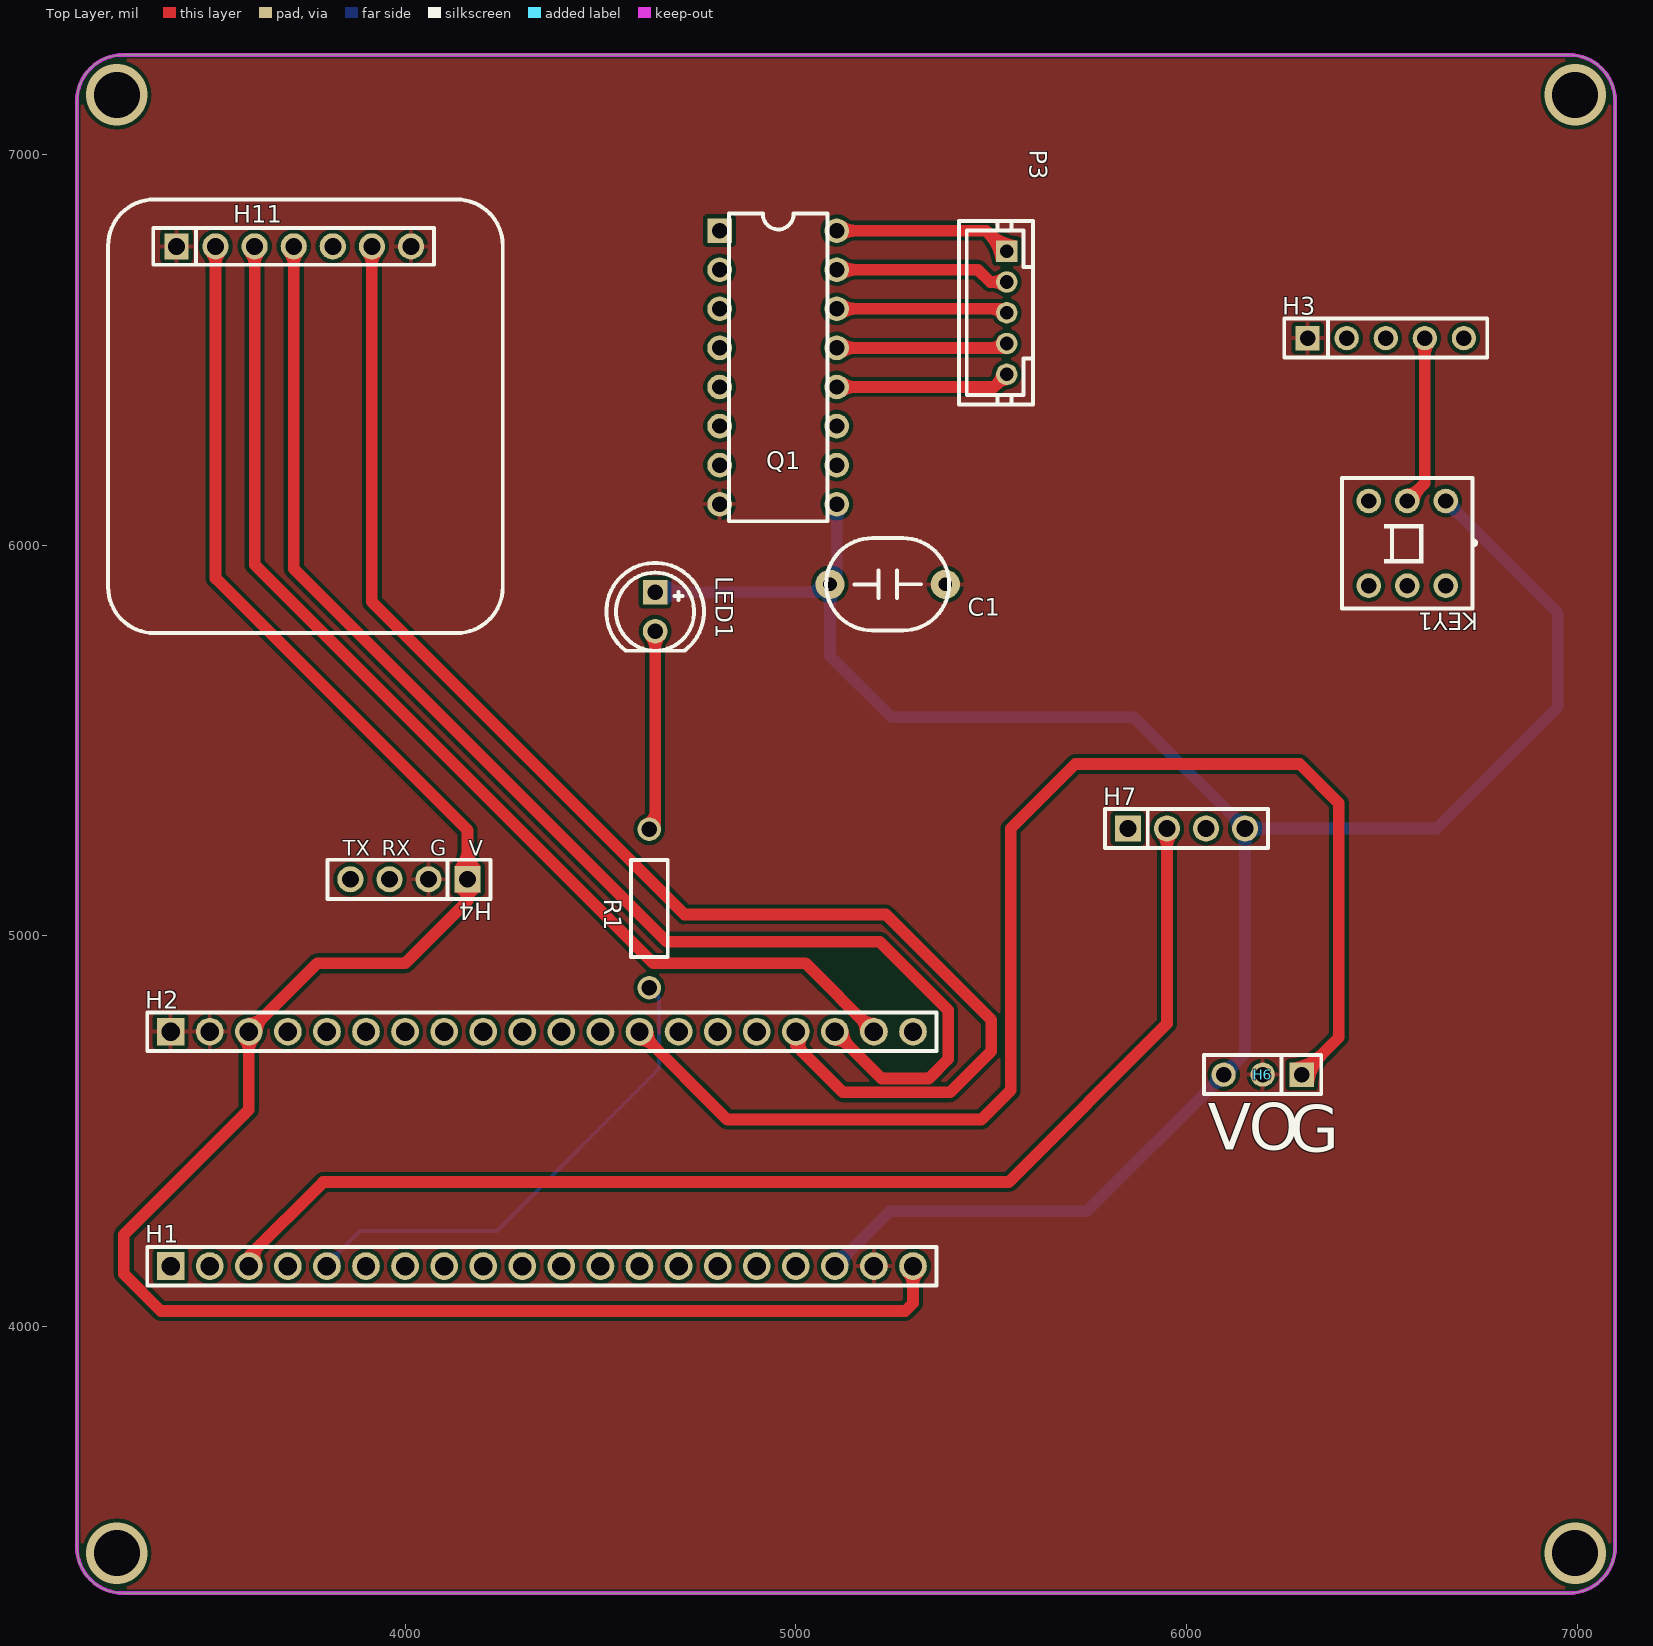
[diagram p0: Top Layer view]
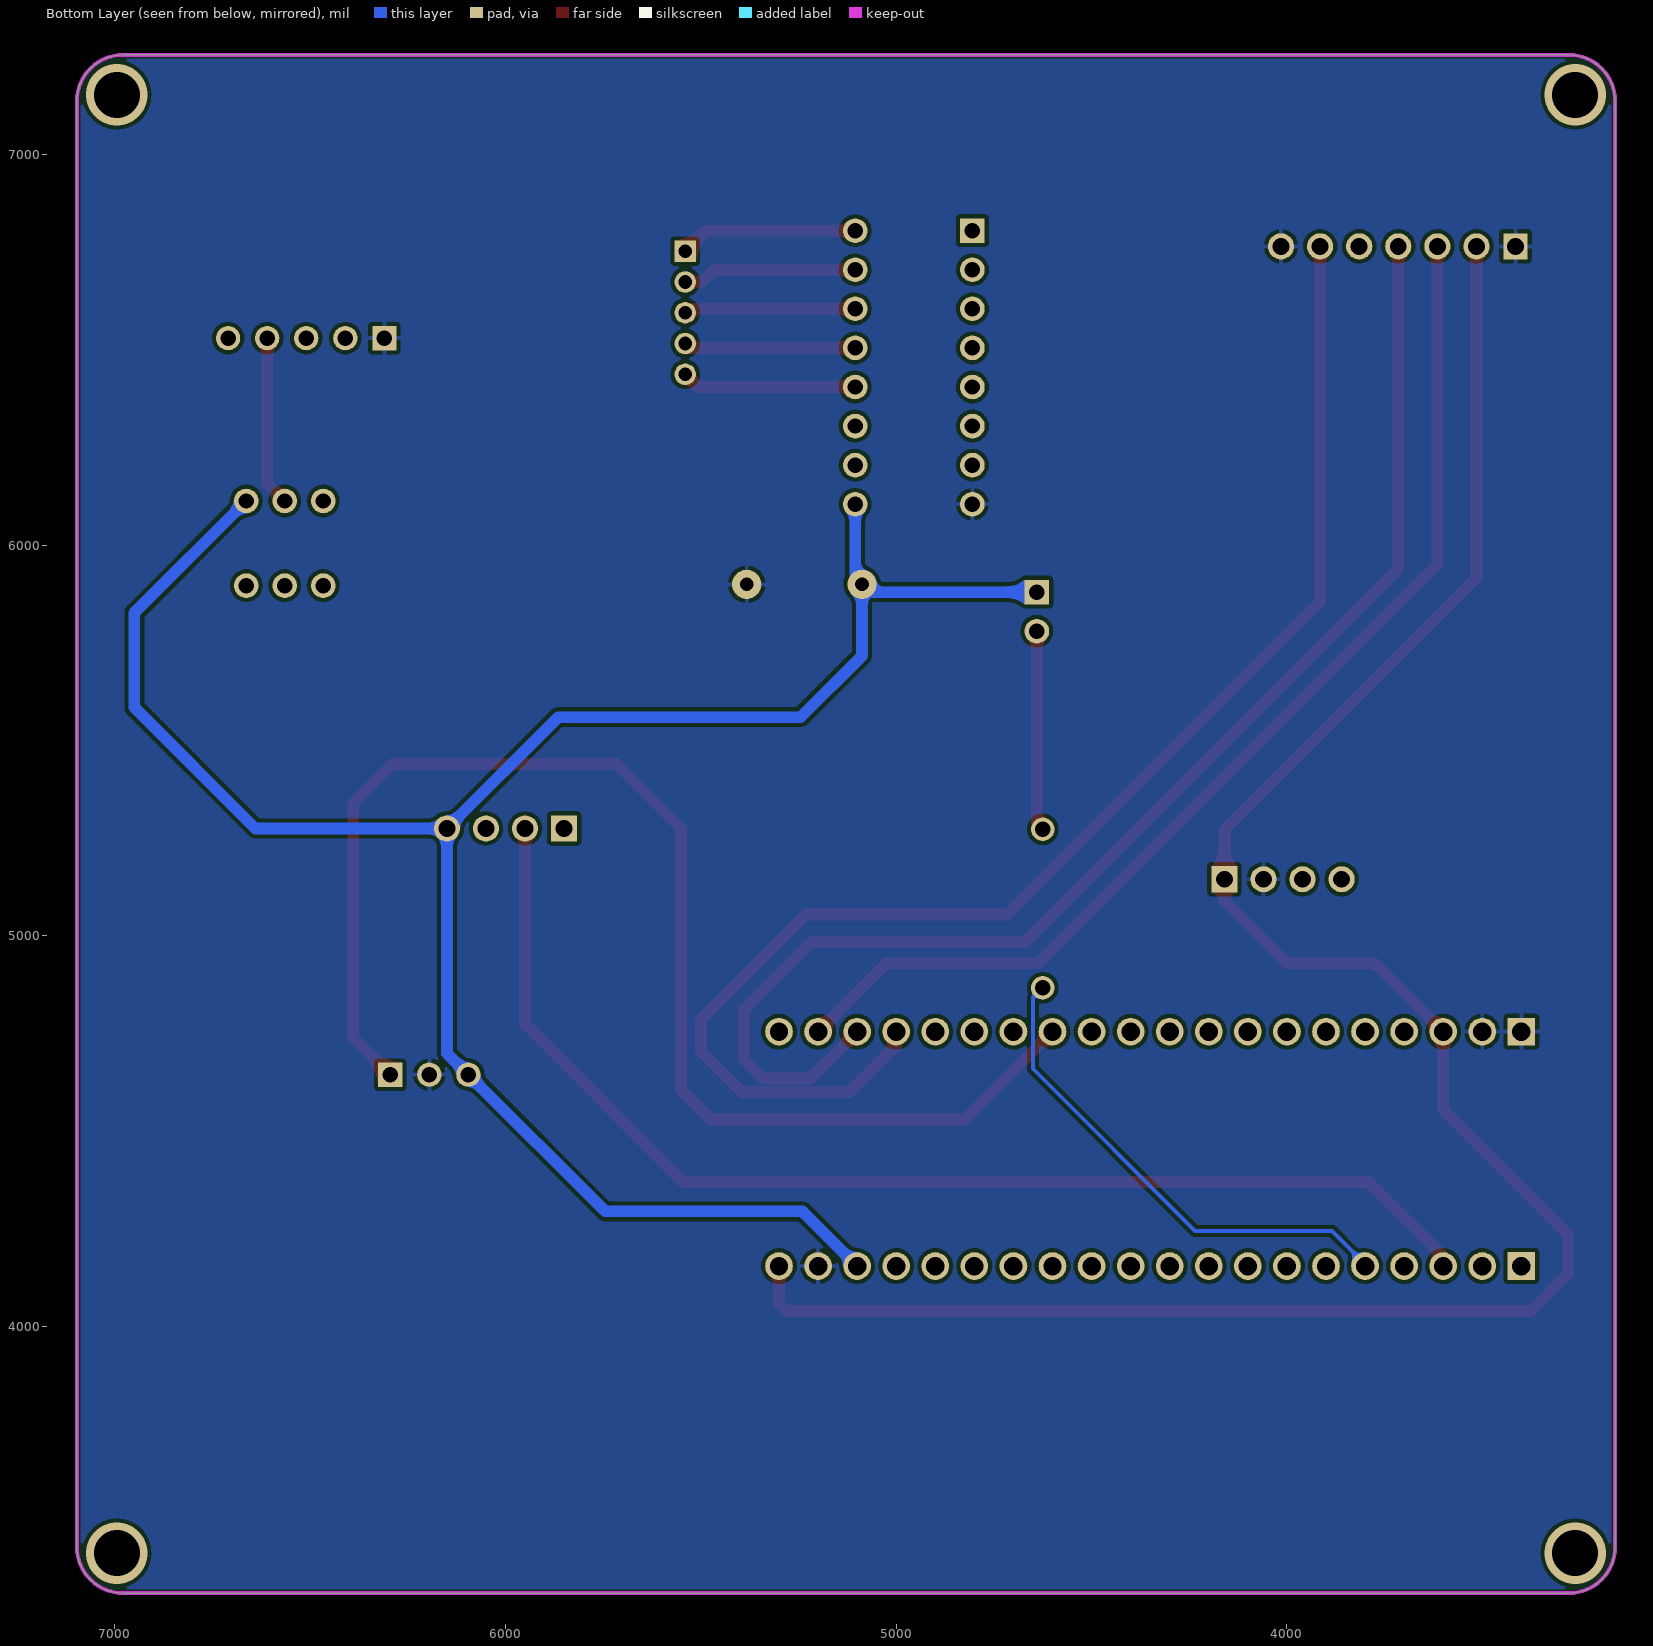
[diagram p1: Bottom Layer view, seen from below]
# Altium PCB MISC89064.pcbdoc
Units mil, origin at the board's own origin, x right, y up, seen from the top; angles counter-clockwise.
Board outline 3937.01 x 3937.01 mil, 2 copper layers (Top Layer, Bottom Layer), stack 62.206 mil thick; 13 components, 49 nets, 96 pads, 4 vias.

## Layer stack, top to bottom
Top Solder Mask Layer: solder mask 0.394, Dk 3.3
Top Layer: signal copper 1.379
Dielectric1: surface 59.449, FR4, Dk 4.5
Bottom Layer: signal copper 1.378
Bottom Solder Mask Layer: solder mask 0.394, Dk 3.3

## Board outline
3278.11,7255 ccw(c3278.11,7136.89) 3160,7136.89 3160,3436.1 ccw(c3278.11,3436.1) 3278.11,3317.99 6978.9,3317.99 ccw(c6978.9,3436.1) 7097.01,3436.1 7097.01,7136.89 ccw(c6978.9,7136.89) 6978.9,7255

## Design rules (kind name [scope] priority, off if disabled: settings)
BoardOutlineClearance copperThickness2oz_1 [All] p2 off: genericclearance=7.99 ignorepadtopadclearanceinfootprint=FALSE except(0: Arc-SplitContinuation Track-SplitContinuation SMDPad-SplitContinuation THPad-SplitContinuation Via-SplitContinuation Fill-SplitContinuation Region-SplitContinuation Poly-SplitContinuation Text-SplitContinuation Hole-SplitContinuation; 5.98: SMDPad-CutoutEdge THPad-CutoutEdge Via-CutoutEdge Fill-CutoutEdge Region-CutoutEdge Text-CutoutEdge Hole-CutoutEdge; 10: Poly-OutlineEdge Poly-CutoutEdge; 11.81: Arc-OutlineEdge Track-OutlineEdge SMDPad-OutlineEdge THPad-OutlineEdge Via-OutlineEdge Fill-OutlineEdge Region-OutlineEdge Text-OutlineEdge Hole-OutlineEdge Arc-CutoutEdge Track-CutoutEdge)
BoardOutlineClearance Plane_innerPlane_1 [All] p4 off: genericclearance=4.02 ignorepadtopadclearanceinfootprint=FALSE except(0: Arc-SplitContinuation Track-SplitContinuation SMDPad-SplitContinuation THPad-SplitContinuation Via-SplitContinuation Fill-SplitContinuation Region-SplitContinuation Poly-SplitContinuation Text-SplitContinuation Hole-SplitContinuation; 5.98: SMDPad-CutoutEdge THPad-CutoutEdge Via-CutoutEdge Fill-CutoutEdge Region-CutoutEdge Text-CutoutEdge Hole-CutoutEdge; 10: Poly-OutlineEdge Poly-CutoutEdge; 11.81: Arc-OutlineEdge Track-OutlineEdge SMDPad-OutlineEdge THPad-OutlineEdge Via-OutlineEdge Fill-OutlineEdge Region-OutlineEdge Text-OutlineEdge Hole-OutlineEdge Arc-CutoutEdge Track-CutoutEdge)
BoardOutlineClearance Copper_copperRegion_1 [All] p6 off: genericclearance=4.02 ignorepadtopadclearanceinfootprint=FALSE except(0: Arc-SplitContinuation Track-SplitContinuation SMDPad-SplitContinuation THPad-SplitContinuation Via-SplitContinuation Fill-SplitContinuation Region-SplitContinuation Poly-SplitContinuation Text-SplitContinuation Hole-SplitContinuation; 5.98: SMDPad-CutoutEdge THPad-CutoutEdge Via-CutoutEdge Fill-CutoutEdge Region-CutoutEdge Text-CutoutEdge Hole-CutoutEdge; 10: Poly-OutlineEdge Poly-CutoutEdge; 11.81: Arc-OutlineEdge Track-OutlineEdge SMDPad-OutlineEdge THPad-OutlineEdge Via-OutlineEdge Fill-OutlineEdge Region-OutlineEdge Text-OutlineEdge Hole-OutlineEdge Arc-CutoutEdge Track-CutoutEdge)
BoardOutlineClearance copperThickness1oz_1 [All] p8: genericclearance=4.02 ignorepadtopadclearanceinfootprint=FALSE except(0: Arc-SplitContinuation Track-SplitContinuation SMDPad-SplitContinuation THPad-SplitContinuation Via-SplitContinuation Fill-SplitContinuation Region-SplitContinuation Poly-SplitContinuation Text-SplitContinuation Hole-SplitContinuation; 5.98: SMDPad-CutoutEdge THPad-CutoutEdge Via-CutoutEdge Fill-CutoutEdge Region-CutoutEdge Text-CutoutEdge Hole-CutoutEdge; 10: Poly-OutlineEdge Poly-CutoutEdge; 11.81: Arc-OutlineEdge Track-OutlineEdge SMDPad-OutlineEdge THPad-OutlineEdge Via-OutlineEdge Fill-OutlineEdge Region-OutlineEdge Text-OutlineEdge Hole-OutlineEdge Arc-CutoutEdge Track-CutoutEdge)
Clearance copperThickness2oz [All] p1 off: gap=7.99 ignorepadtopadclearanceinfootprint=FALSE except(5.98: SMDPad-Track SMDPad-SMDPad THPad-Track SMDPad-THPad THPad-THPad Track-Via SMDPad-Via THPad-Via Via-Via Fill-Track Region-Track Fill-SMDPad Region-SMDPad Fill-THPad Region-THPad Fill-Via Region-Via Fill-Fill Fill-Region Region-Region Arc-Track Arc-SMDPad Arc-THPad Arc-Via Fill-Arc Region-Arc Arc-Arc Text-Track SMDPad-Text Text-THPad Text-Via Fill-Text Region-Text Arc-Text Text-Text Hole-Track Hole-SMDPad Hole-THPad Hole-Via Fill-Hole Region-Hole Hole-Arc Hole-Text; 10: Poly-Track Poly-SMDPad Poly-THPad Poly-Via Poly-Fill Poly-Region Poly-Poly Poly-Arc Poly-Text Poly-Hole)
Clearance Plane_innerPlane [All] p3 off: gap=4.02 ignorepadtopadclearanceinfootprint=FALSE except(5.98: SMDPad-Track SMDPad-SMDPad THPad-Track SMDPad-THPad THPad-THPad Track-Via SMDPad-Via THPad-Via Via-Via Fill-Track Region-Track Fill-SMDPad Region-SMDPad Fill-THPad Region-THPad Fill-Via Region-Via Fill-Fill Fill-Region Region-Region Arc-Track Arc-SMDPad Arc-THPad Arc-Via Fill-Arc Region-Arc Arc-Arc Text-Track SMDPad-Text Text-THPad Text-Via Fill-Text Region-Text Arc-Text Text-Text Hole-Track Hole-SMDPad Hole-THPad Hole-Via Fill-Hole Region-Hole Hole-Arc Hole-Text; 10: Poly-Track Poly-SMDPad Poly-THPad Poly-Via Poly-Fill Poly-Region Poly-Poly Poly-Arc Poly-Text Poly-Hole)
Clearance Copper_copperRegion [All] p5 off: gap=4.02 ignorepadtopadclearanceinfootprint=FALSE except(5.98: SMDPad-Track SMDPad-SMDPad THPad-Track SMDPad-THPad THPad-THPad Track-Via SMDPad-Via THPad-Via Via-Via Fill-Track Region-Track Fill-SMDPad Region-SMDPad Fill-THPad Region-THPad Fill-Via Region-Via Fill-Fill Fill-Region Region-Region Arc-Track Arc-SMDPad Arc-THPad Arc-Via Fill-Arc Region-Arc Arc-Arc Text-Track SMDPad-Text Text-THPad Text-Via Fill-Text Region-Text Arc-Text Text-Text Hole-Track Hole-SMDPad Hole-THPad Hole-Via Fill-Hole Region-Hole Hole-Arc Hole-Text; 10: Poly-Track Poly-SMDPad Poly-THPad Poly-Via Poly-Fill Poly-Region Poly-Poly Poly-Arc Poly-Text Poly-Hole)
Clearance copperThickness1oz [All] p7: gap=4.02 ignorepadtopadclearanceinfootprint=FALSE except(5.98: SMDPad-Track SMDPad-SMDPad THPad-Track SMDPad-THPad THPad-THPad Track-Via SMDPad-Via THPad-Via Via-Via Fill-Track Region-Track Fill-SMDPad Region-SMDPad Fill-THPad Region-THPad Fill-Via Region-Via Fill-Fill Fill-Region Region-Region Arc-Track Arc-SMDPad Arc-THPad Arc-Via Fill-Arc Region-Arc Arc-Arc Text-Track SMDPad-Text Text-THPad Text-Via Fill-Text Region-Text Arc-Text Text-Text Hole-Track Hole-SMDPad Hole-THPad Hole-Via Fill-Hole Region-Hole Hole-Arc Hole-Text; 10: Poly-Track Poly-SMDPad Poly-THPad Poly-Via Poly-Fill Poly-Region Poly-Poly Poly-Arc Poly-Text Poly-Hole)
DiffPairsRouting differentialPair [All] p1: maxlimit=6 minlimit=6 mostfreqgap=6 toplayer_minwidth=5 toplayer_prefwidth=10 toplayer_maxwidth=100 toplayer_mingap=6 toplayer_prefgap=6 toplayer_maxgap=6 bottomlayer_minwidth=5 bottomlayer_prefwidth=10 bottomlayer_maxwidth=100 bottomlayer_mingap=6 bottomlayer_prefgap=6 bottomlayer_maxgap=6 maxuncoupledlength=10
HoleToHoleClearance otherClearance [All] p1: gap=11.8 allowstackedmicrovias=TRUE
Length netLength [All] p1: minlimit=0 maxlimit=0
PasteMaskExpansion pasteMaskExpansion [All] p1: expansion=0
PlaneConnect innerPlane [All] p1: planeconnectstyle=Relief reliefexpansion=20 reliefentries=4 reliefconductorwidth=10 reliefairgap=10
PolygonConnect copperRegion [All] p1: connectstyle=Relief reliefconductorwidth=10 reliefentries=4 polygonreliefangle="90 Angle" airgapwidth=10 via.connectstyle=Relief via.reliefconductorwidth=10 via.reliefentries=4 via.polygonreliefangle="90 Angle" via.airgapwidth=10
RoutingVias viaSize [All] p1: holewidth=12.01 width=24.02 viastyle="Through Hole" minholewidth=11.81 minwidth=19.68 maxholewidth=248.03 maxwidth=393.7
SolderMaskExpansion solderMaskExpansion [IsVia] p1: expansion=-1000 istentingtop=TRUE
SolderMaskExpansion solderMaskExpansion [All] p2: expansion=2 istentingtop=FALSE
Width copperThickness2oz_2 [All] p1 off: maxlimit=100 minlimit=8 preferedwidth=10
Width copperThickness1oz_2 [All] p2: maxlimit=100 minlimit=5 preferedwidth=10

## Components (designator, comment, footprint, x,y, rotation, side; value= is the part's Value field where it differs from the comment)
C1 "10pF" CAP-TH_L5.5-W6.0-P7.50-D0.6 5235,5900 r0 top
H1 "" HDR-TH_20P-P2.54-V-F 4350,4155 r0 top
H2 "" HDR-TH_20P-P2.54-V-F 4350,4755 r0 top
H3 "" HDR-TH_5P-P2.54-V-F 6510,6530 r0 top
H4 "" HDR-TH_4P-P2.54-V-F 4010,5145 r180 top
H6 "" HDR-TH_3P-P2.54-V-F 6195,4645 r180 top
H7 "" HDR-TH_4P-P2.54-V-F 6000,5275 r0 top
H11 "" HDR-TH_7P-P2.54-V-F 3715,6765 r0 top
KEY1 "Non-self-locking switch 8.5×8.5 silent" SW-TH_6P-L8.5-W8.5-P2.54 6565,6005 r180 top
LED1 "" LED_TH-_5mm 4640,5830 r270 top
P3 "PH2.0_5P through-hole socket" CONN-TH_5P-P2.00-PH5A 5540,6595 r270 top
Q1 "ULN2003" DIP-16_L19.8-W6.5-P2.54-LS7.6-BL 4955,6455 r270 top
R1 "1k" Res_1/4W 4625,5070 r90 top

## Footprints (in the part's own frame and the unit in brackets; to place one, negate y for a bottom-side part, rotate by r counter-clockwise, add the part's x,y. Pads: shape width x height; smd on the part's side, far side on the other; paste and mask are expansions set on the pad)
CAP-TH_L5.5-W6.0-P7.50-D0.6 [mm]
  round 1.9 hole 0.9 paste+0 mask+0.05: 1(-3.75,0) 2(3.75,0)
  silkscreen extent -4,-3 4,3
CONN-TH_5P-P2.00-PH5A [mm]
  rect 1.4x1.4 hole 0.9: 1(-4,0)
  round 1.4 hole 0.9: 2(-2,0) 3(0,0) 4(2,0) 5(4,0)
  silkscreen extent -5.96,-3.1 5.96,1.7
DIP-16_L19.8-W6.5-P2.54-LS7.6-BL [mm]
  rect 1.6x1.6 hole 1: 1(-8.89,-3.81)
  round 1.6 hole 1 copper offset 0,0: 2(-6.35,-3.81) 3(-3.81,-3.81) 4(-1.27,-3.81) 5(1.27,-3.81) 6(3.81,-3.81) 7(6.35,-3.81) 8(8.89,-3.81) 9(8.89,3.81) 10(6.35,3.81) 11(3.81,3.81) 12(1.27,3.81) 13(-1.27,3.81) 14(-3.81,3.81) 15(-6.35,3.81) 16(-8.89,3.81)
  silkscreen extent -10,-3.2 10,3.2
HDR-TH_3P-P2.54-V-F [mil]
  rect 62x62 hole 40.16: 1(-100,0)
  round 62 hole 40.16: 2(0,0) 3(100,0)
  silkscreen extent -150,-50 150,50
HDR-TH_4P-P2.54-V-F [mm]
  rect 1.7x1.7 hole 1.1: 1(-3.81,0)
  round 1.7 hole 1.1: 2(-1.27,0) 3(1.27,0) 4(3.81,0)
  silkscreen extent -5.29,-1.27 5.29,1.27
HDR-TH_5P-P2.54-V-F [mil]
  rect 62x62 hole 40.16: 1(-200,0)
  round 62 hole 40.16: 2(-100,0) 3(0,0) 4(100,0) 5(200,0)
  silkscreen extent -260,-50 260,50
HDR-TH_7P-P2.54-V-F [mm]
  rect 1.575x1.7 hole 1.1: 1(-7.62,0)
  round 1.7 hole 1.1: 2(-5.08,0) 3(-2.54,0) 4(0,0) 5(2.54,0) 6(5.08,0) 7(7.62,0)
  silkscreen extent -9.13,-1.2 9.13,1.2
HDR-TH_20P-P2.54-V-F [mm]
  rect 1.8x1.8 hole 1.2: 1(-24.13,0)
  round 1.8 hole 1.2: 2(-21.59,0) 3(-19.05,0) 4(-16.51,0) 5(-13.97,0) 6(-11.43,0) 7(-8.89,0) 8(-6.35,0) 9(-3.81,0) 10(-1.27,0) 11(1.27,0) 12(3.81,0) 13(6.35,0) 14(8.89,0) 15(11.43,0) 16(13.97,0) 17(16.51,0) 18(19.05,0) 19(21.59,0) 20(24.13,0)
  silkscreen extent -25.65,-1.25 25.65,1.25
LED_TH-_5mm [mm]
  rect 1.6x1.6 hole 1 paste+0 mask+0.051: 1(-1.27,0)
  round 1.6 hole 1 paste+0 mask+0.051: 2(1.27,0)
  silkscreen extent -3.17,-3.17 2.54,3.17
Res_1/4W [mil]
  round 60 hole 39.37 paste+0 mask+2: 1(-202.76,0) 2(202.76,0)
  silkscreen extent -124,-47 124,47
SW-TH_6P-L8.5-W8.5-P2.54 [mm]
  round 1.6 hole 1: 1(-2.5,-2.75) 2(0,-2.75) 3(2.5,-2.75) 4(-2.5,2.75) 5(0,2.75) 6(2.5,2.75)
  silkscreen extent -4.47,-4.25 4.25,4.25

## Via types
v1: diameter 157.48, hole 118.1, Top Layer to Bottom Layer, 4 vias

## Nets (pads, with @x,y where several pads share a name; then routed paths per layer and width w, separated by ;. In a path a pad name is that pad's centre, name@x,y a point inside that pad or via, vN(x,y) a via of type N, cw(c..) or ccw(c..) an arc to the next point about the centre after c; other vN are vias at no path point)
$1N5862: LED1.2 R1.2 | length 513.5
  Top Layer w30: R1.2 4640,5287.76 LED1.2
$1N6179: P3.1 Q1.16 | length 456.8
  Top Layer w30: Q1.16 5487.48,6805 P3.1
$1N6181: P3.2 Q1.15 | length 447.9
  Top Layer w30: Q1.15 5466.18,6705 5497.44,6673.74 P3.2
$1N6183: P3.3 Q1.14 | length 439.1
  Top Layer w30: Q1.14 5530,6605 P3.3
$1N6185: P3.4 Q1.13 | length 439.7
  Top Layer w30: Q1.13 5528.74,6505 P3.4
$1N6195: P3.5 Q1.12 | length 448.5
  Top Layer w30: Q1.12 5507.48,6405 P3.5
+5V: C1.1 H1.18 H6.3 H7.4 KEY1.1 LED1.1 Q1.9 | length 5522.4
  Bottom Layer w30: LED1.1 5067.36,5880 C1.1 ; H1.18 5240,4295 5745,4295 H6.3 6150,4700 H7.4 ; Q1.9 5105,5917.64 C1.1 ; KEY1.1 6950,5826.69 6950,5585 6640,5275 H7.4 ; C1.1 5087.36,5717.64 5245,5560 5865,5560 H7.4
+5V1: H3.4 KEY1.2 | length 435.4
  Top Layer w30: KEY1.2 6610,6158.27 H3.4
GND: C1.2 H1.19 H2.1 H2.2 H3.1 H4.2 H6.2 H11.1 H11.7 Q1.8
PA0: H2.16
PA1: H2.15
PA2: H2.14
PA3: H2.13 H6.1 | length 3428.4
  Top Layer w30: H2.13 4825,4530 5475,4530 5550,4605 5550,5275 5715,5440 6290,5440 6390,5340 6390,4740 H6.1
PA4: H2.12
PA5: H2.11
PA6: H2.10
PA7: H2.9
PA8: H1.5 R1.1 | length 1279.7
  Bottom Layer w10: H1.5 3800,4160 3885,4245 4235,4245 4650,4660 4650,4842.24 R1.1
PA9: H1.6
PA10: H1.7
PA11: H1.8
PA12: H1.9
PA15: H1.10
PB0: H2.8
PB1: H2.7
PB3: H1.11
PB4: H1.12
PB5: H1.13
PB6: H1.14
PB7: H11.5
PB10: H2.6
PB11: H2.5
PB12: H1.1
PB13: H1.2
PB14: H1.3 H7.2 | length 3121.5
  Top Layer w30: H1.3 3600,4180 3790,4370 5545,4370 5950,4775 H7.2
PB15: H1.4
PC13: H2.19 H11.3 | length 2895
  Top Layer w30: H11.3 3615,5950 4635,4930 5025,4930 H2.19
PC14: H2.18 H11.4 | length 3453.5
  Top Layer w30: H11.4 3715,5940 4670,4985 5215,4985 5390,4810 5390,4685 5340,4635 5220,4635 H2.18
PC15: H2.17 H11.6 | length 3646.4
  Top Layer w30: H11.6 3915,5855 4715,5055 5230,5055 5500,4785 5500,4705 5395,4600 5120,4600 5000,4720 H2.17
PC20: Q1.1
PC21: Q1.2
PC22: Q1.3
PC23: Q1.4
RES: H1.15
RXD: H4.3
SCL: H1.17
SDA: H1.16
TXD: H4.4
VCC: H1.20 H2.3 H4.1 H11.2 | length 5556.1
  Top Layer w30: H11.2 3515,5915 4160,5270 H4.1 4160,5090 4000,4930 3775,4930 H2.3 3600,4555 3280,4235 3280,4135 3375,4040 5280,4040 5300,4060 H1.20
pads on no net: H2.4 H2.20 H3.2 H3.3 H3.5 H7.1 H7.3 KEY1.3 KEY1.4 KEY1.5 KEY1.6 Q1.5 Q1.6 Q1.7 Q1.10 Q1.11
copper on no net:
  other v1: 3262.36,3420.35 6994.65,3420.35 3262.36,7152.64 6994.65,7152.64

## Polygon pours and split planes (outlines as drawn)
GND on Top Layer (solid, remove dead copper, pour order 0): 3080,7375 3080,3020 7440,3020 7440,7375
GND on Bottom Layer (solid, remove dead copper, pour order 4): 3000,7505 3000,3000 7520,3000 7520,7505

## Keep-outs
Board Outline Layer:
  the board outline again, w10

## Other copper
Top Layer:
  region net VCC: 3644.72,4778.5 3623.5,4799.72 3622.29,4798.6 3620.98,4797.56 3619.58,4796.6 3618.1,4795.72 3616.56,4794.92 3614.13,4793.84 3611.6,4792.93 3609,4792.16 3606.37,4791.53 3602.87,4790.9 3599.44,4790.49 3597.78,4790.36 3635.36,4752.78 3635.67,4756.14 3636.19,4759.61 3636.93,4763.13 3637.65,4765.74 3638.52,4768.29 3639.54,4770.76 3640.31,4772.34 3641.15,4773.85 3642.07,4775.29 3643.07,4776.65 3644.15,4777.91
  region net VCC: 4145,5090 4175,5090 4175.34,5093.84 4176.35,5097.56 4178.01,5101.05 4180.25,5104.18 4183.01,5106.88 4186.2,5109.04 4189.72,5110.61 4193.46,5111.54 4126.54,5111.54 4130.28,5110.61 4133.8,5109.04 4136.99,5106.88 4139.75,5104.18 4141.99,5101.05 4143.65,5097.56 4144.66,5093.84
  region net $1N6179: 5147.88,6790 5147.88,6820 5146.61,6820.05 5145.26,6820.19 5143.11,6820.57 5140.86,6821.13 5138.56,6821.85 5135.48,6823 5132.51,6824.35 5130.42,6825.46 5128.51,6826.62 5127.35,6827.41 5126.31,6828.22 5125.83,6828.62 5125.83,6781.38 5126.81,6782.19 5127.92,6782.99 5129.76,6784.16 5131.8,6785.29 5133.98,6786.34 5137.01,6787.6 5139.33,6788.41 5141.62,6789.07 5143.84,6789.57 5145.26,6789.81 5146.61,6789.95
  region net $1N6179: 5501.83,6811.86 5480.62,6790.65 5486.76,6784 5492.34,6776.88 5497.33,6769.33 5501.69,6761.41 5505.41,6753.16 5508.45,6744.64 5510.8,6735.9 5512.44,6727.01 5565.47,6780.04 5556.58,6781.68 5547.84,6784.03 5539.32,6787.07 5531.07,6790.79 5523.15,6795.15 5515.6,6800.14 5508.48,6805.72 5501.83,6811.86
  region net $1N6181: 5147.88,6690 5147.88,6720 5146.61,6720.05 5145.26,6720.19 5143.11,6720.57 5140.86,6721.13 5138.56,6721.85 5135.48,6723 5132.51,6724.35 5130.42,6725.46 5128.51,6726.62 5127.35,6727.41 5126.31,6728.22 5125.83,6728.62 5125.83,6681.38 5126.81,6682.19 5127.92,6682.99 5129.76,6684.16 5131.8,6685.29 5133.98,6686.34 5137.01,6687.6 5139.33,6688.41 5141.62,6689.07 5143.84,6689.57 5145.26,6689.81 5146.61,6689.95
  region net $1N6181: 5502.48,6688.74 5502.48,6658.74 5504.96,6658.67 5507.53,6658.45 5510.14,6658.07 5512.09,6657.66 5514,6657.14 5515.85,6656.51 5517.05,6656.02 5518.2,6655.47 5519.29,6654.86 5520.33,6654.19 5521.31,6653.46 5521.77,6653.07 5521.77,6694.41 5520.83,6693.64 5519.82,6692.94 5518.75,6692.31 5517.63,6691.73 5516.46,6691.21 5514.62,6690.53 5512.73,6689.98 5510.79,6689.54 5508.83,6689.2 5506.24,6688.9 5503.7,6688.76
  region net $1N6183: 5147.88,6590 5147.88,6620 5146.61,6620.05 5145.26,6620.19 5143.11,6620.57 5140.86,6621.13 5138.56,6621.85 5135.48,6623 5132.51,6624.35 5130.42,6625.46 5128.51,6626.62 5127.35,6627.41 5126.31,6628.22 5125.83,6628.62 5125.83,6581.38 5126.81,6582.19 5127.92,6582.99 5129.76,6584.16 5131.8,6585.29 5133.98,6586.34 5137.01,6587.6 5139.33,6588.41 5141.62,6589.07 5143.84,6589.57 5145.26,6589.81 5146.61,6589.95
  region net $1N6183: 5502.48,6620 5502.48,6590 5504.06,6589.95 5505.02,6589.86 5505.92,6589.73 5506.75,6589.56 5507.53,6589.35 5508.25,6589.1 5508.92,6588.81 5509.55,6588.49 5510.14,6588.13 5510.68,6587.75 5511.2,6587.33 5511.69,6586.88 5512.15,6586.41 5512.81,6585.64 5513.65,6584.54 5516.2,6580.77 5517.71,6578.69 5518.88,6577.25 5520.22,6575.8 5521.36,6574.7 5521.77,6574.33 5521.77,6615.67 5521.33,6615.33 5520.87,6615.06 5520.39,6614.85 5519.89,6614.71 5519.37,6614.62 5518.82,6614.58 5518.27,6614.6 5517.69,6614.66 5517.11,6614.76 5515.89,6615.08 5514.64,6615.51 5512.69,6616.33 5508.06,6618.48 5506.12,6619.26 5504.86,6619.65 5504.25,6619.8 5503.64,6619.91 5503.05,6619.98
  region net $1N6185: 5147.88,6490 5147.88,6520 5146.61,6520.05 5145.26,6520.19 5143.11,6520.57 5140.86,6521.13 5138.56,6521.85 5135.48,6523 5132.51,6524.35 5130.42,6525.46 5128.51,6526.62 5127.35,6527.41 5126.31,6528.22 5125.83,6528.62 5125.83,6481.38 5126.81,6482.19 5127.92,6482.99 5129.76,6484.16 5131.8,6485.29 5133.98,6486.34 5137.01,6487.6 5139.33,6488.41 5141.62,6489.07 5143.84,6489.57 5145.26,6489.81 5146.61,6489.95
  region net $1N6185: 5502.48,6520 5502.48,6490 5503.09,6490.03 5503.7,6490.11 5504.32,6490.24 5504.95,6490.41 5506.23,6490.88 5507.52,6491.47 5510.13,6492.89 5514,6495.08 5515.25,6495.68 5516.46,6496.17 5517.05,6496.36 5517.63,6496.51 5518.2,6496.6 5518.76,6496.65 5519.3,6496.64 5519.83,6496.57 5520.34,6496.43 5520.83,6496.23 5521.31,6495.95 5521.77,6495.59 5521.77,6536.93 5520.5,6535.74 5519.38,6534.56 5518.4,6533.38 5517.26,6531.84 5516.05,6529.98 5513.89,6526.21 5513.13,6525 5512.54,6524.15 5512.12,6523.62 5511.68,6523.12 5511.2,6522.66 5510.69,6522.22 5510.14,6521.82 5509.54,6521.45 5508.9,6521.13 5508.19,6520.84 5507.42,6520.59 5506.59,6520.38 5505.68,6520.22 5504.7,6520.1 5503.07,6520.01
  region net $1N6195: 5147.88,6390 5147.88,6420 5146.61,6420.05 5145.26,6420.19 5143.11,6420.57 5140.86,6421.13 5138.56,6421.85 5135.48,6423 5132.51,6424.35 5130.42,6425.46 5128.51,6426.62 5127.35,6427.41 5126.31,6428.22 5125.83,6428.62 5125.83,6381.38 5126.81,6382.19 5127.92,6382.99 5129.76,6384.16 5131.8,6385.29 5133.98,6386.34 5137.01,6387.6 5139.33,6388.41 5141.62,6389.07 5143.84,6389.57 5145.26,6389.81 5146.61,6389.95
  region net $1N6195: 5502.86,6421.6 5524.08,6400.38 5525.88,6402.09 5527.85,6403.75 5529.97,6405.32 5531.63,6406.41 5533.35,6407.4 5535.11,6408.26 5536.3,6408.76 5537.5,6409.18 5538.71,6409.53 5539.92,6409.79 5541.12,6409.96 5541.73,6410.02 5512.5,6439.25 5512.37,6438.04 5512.15,6436.83 5511.85,6435.62 5511.46,6434.42 5511,6433.22 5510.18,6431.45 5509.23,6429.72 5508.18,6428.03 5507.03,6426.41 5505.41,6424.36 5503.72,6422.47
  region net VCC: 3500,6719.44 3530,6719.44 3530.06,6720.9 3530.23,6722.4 3530.5,6723.95 3530.87,6725.52 3531.58,6727.9 3532.48,6730.29 3533.52,6732.65 3534.68,6734.95 3535.95,6737.16 3537.29,6739.23 3538.68,6741.15 3540.1,6742.87 3489.9,6742.87 3491.32,6741.15 3492.71,6739.23 3494.05,6737.16 3495.32,6734.95 3496.48,6732.65 3497.52,6730.29 3498.42,6727.9 3499.13,6725.52 3499.5,6723.95 3499.77,6722.4 3499.94,6720.9
  region net VCC: 4175,5223.46 4145,5223.46 4144.6,5216.35 4143.42,5209.33 4141.46,5202.48 4138.76,5195.89 4135.34,5189.64 4131.25,5183.81 4126.54,5178.46 4193.46,5178.46 4188.75,5183.81 4184.66,5189.64 4181.24,5195.89 4178.54,5202.48 4176.58,5209.33 4175.4,5216.35 4175,5223.46
  region net PC13: 3600,6719.44 3630,6719.44 3630.06,6720.9 3630.23,6722.4 3630.5,6723.95 3630.87,6725.52 3631.58,6727.9 3632.48,6730.29 3633.52,6732.65 3634.68,6734.95 3635.95,6737.16 3637.29,6739.23 3638.68,6741.15 3640.1,6742.87 3589.9,6742.87 3591.32,6741.15 3592.71,6739.23 3594.05,6737.16 3595.32,6734.95 3596.48,6732.65 3597.52,6730.29 3598.42,6727.9 3599.13,6725.52 3599.5,6723.95 3599.77,6722.4 3599.94,6720.9
  region net PC13: 5176.5,4799.72 5155.28,4778.5 5156.4,4777.29 5157.44,4775.98 5158.4,4774.58 5159.28,4773.1 5160.08,4771.56 5161.16,4769.13 5162.07,4766.6 5162.84,4764 5163.47,4761.37 5164.1,4757.87 5164.51,4754.44 5164.64,4752.78 5202.22,4790.36 5198.86,4790.67 5195.39,4791.19 5191.87,4791.93 5189.26,4792.65 5186.71,4793.52 5184.24,4794.54 5182.66,4795.31 5181.15,4796.15 5179.71,4797.07 5178.35,4798.07 5177.09,4799.15
  region net PC14: 5123.5,4710.28 5144.72,4731.5 5143.6,4732.71 5142.56,4734.02 5141.6,4735.42 5140.72,4736.9 5139.92,4738.44 5138.84,4740.87 5137.93,4743.4 5137.16,4746 5136.53,4748.63 5135.9,4752.13 5135.49,4755.56 5135.36,4757.22 5097.78,4719.64 5101.14,4719.33 5104.61,4718.81 5108.13,4718.07 5110.74,4717.35 5113.29,4716.48 5115.76,4715.46 5117.34,4714.69 5118.85,4713.85 5120.29,4712.93 5121.65,4711.93 5122.91,4710.85
  region net PC15: 3900,6719.44 3930,6719.44 3930.06,6720.9 3930.23,6722.4 3930.5,6723.95 3930.87,6725.52 3931.58,6727.9 3932.48,6730.29 3933.52,6732.65 3934.68,6734.95 3935.95,6737.16 3937.29,6739.23 3938.68,6741.15 3940.1,6742.87 3889.9,6742.87 3891.32,6741.15 3892.71,6739.23 3894.05,6737.16 3895.32,6734.95 3896.48,6732.65 3897.52,6730.29 3898.42,6727.9 3899.13,6725.52 3899.5,6723.95 3899.77,6722.4 3899.94,6720.9
  region net PC15: 5006,4692.78 5027.22,4714 5026.78,4714.46 5026.39,4714.94 5026.03,4715.43 5025.72,4715.93 5025.44,4716.45 5025.2,4716.98 5024.99,4717.52 5024.82,4718.08 5024.67,4718.65 5024.57,4719.22 5024.49,4719.81 5024.42,4721.03 5024.46,4722.28 5024.6,4723.57 5024.83,4724.89 5025.33,4726.93 5025.99,4729.03 5027.36,4732.64 5031.9,4743.08 5033.36,4746.79 5034.32,4749.69 5034.86,4751.83 5035.13,4753.22 5035.31,4754.58 5035.39,4755.92 5035.36,4757.22 4997.78,4719.64 4998.66,4719.52 4999.43,4719.31 5000.11,4719 5000.69,4718.59 5001.2,4718.1 5001.62,4717.53 5001.97,4716.88 5002.26,4716.17 5002.49,4715.39 5002.67,4714.55 5002.89,4712.72 5002.98,4709.68 5002.94,4703.1 5003.05,4700.92 5003.29,4698.82 5003.49,4697.82 5003.73,4696.85 5004.04,4695.93 5004.41,4695.05 5004.86,4694.24 5005.39,4693.48
  region net PC15: 3900,6719.44 3930,6719.44 3930.06,6720.9 3930.23,6722.4 3930.5,6723.95 3930.87,6725.52 3931.58,6727.9 3932.48,6730.29 3933.52,6732.65 3934.68,6734.95 3935.95,6737.16 3937.29,6739.23 3938.68,6741.15 3940.1,6742.87 3889.9,6742.87 3891.32,6741.15 3892.71,6739.23 3894.05,6737.16 3895.32,6734.95 3896.48,6732.65 3897.52,6730.29 3898.42,6727.9 3899.13,6725.52 3899.5,6723.95 3899.77,6722.4 3899.94,6720.9
  region net PC14: 3700,6719.44 3730,6719.44 3730.06,6720.9 3730.23,6722.4 3730.5,6723.95 3730.87,6725.52 3731.58,6727.9 3732.48,6730.29 3733.52,6732.65 3734.68,6734.95 3735.95,6737.16 3737.29,6739.23 3738.68,6741.15 3740.1,6742.87 3689.9,6742.87 3691.32,6741.15 3692.71,6739.23 3694.05,6737.16 3695.32,6734.95 3696.48,6732.65 3697.52,6730.29 3698.42,6727.9 3699.13,6725.52 3699.5,6723.95 3699.77,6722.4 3699.94,6720.9
  region net PC13: 5176.5,4799.72 5155.28,4778.5 5156.4,4777.29 5157.44,4775.98 5158.4,4774.58 5159.28,4773.1 5160.08,4771.56 5161.16,4769.13 5162.07,4766.6 5162.84,4764 5163.47,4761.37 5164.1,4757.87 5164.51,4754.44 5164.64,4752.78 5202.22,4790.36 5198.86,4790.67 5195.39,4791.19 5191.87,4791.93 5189.26,4792.65 5186.71,4793.52 5184.24,4794.54 5182.66,4795.31 5181.15,4796.15 5179.71,4797.07 5178.35,4798.07 5177.09,4799.15
  region net PC13: 3600,6719.44 3630,6719.44 3630.06,6720.9 3630.23,6722.4 3630.5,6723.95 3630.87,6725.52 3631.58,6727.9 3632.48,6730.29 3633.52,6732.65 3634.68,6734.95 3635.95,6737.16 3637.29,6739.23 3638.68,6741.15 3640.1,6742.87 3589.9,6742.87 3591.32,6741.15 3592.71,6739.23 3594.05,6737.16 3595.32,6734.95 3596.48,6732.65 3597.52,6730.29 3598.42,6727.9 3599.13,6725.52 3599.5,6723.95 3599.77,6722.4 3599.94,6720.9
  region net $1N5862: 4625,5737.12 4655,5737.12 4655.05,5738.39 4655.19,5739.74 4655.57,5741.89 4656.13,5744.14 4656.85,5746.44 4658,5749.52 4659.35,5752.49 4660.46,5754.58 4661.62,5756.49 4662.41,5757.65 4663.22,5758.69 4663.62,5759.17 4616.38,5759.17 4617.19,5758.19 4617.99,5757.08 4619.16,5755.24 4620.29,5753.2 4621.34,5751.02 4622.6,5747.99 4623.41,5745.67 4624.07,5743.38 4624.57,5741.16 4624.81,5739.74 4624.95,5738.39
  region net $1N5862: 4655,5313.6 4625,5313.6 4624.95,5312.81 4624.81,5312.04 4624.58,5311.27 4624.26,5310.52 4623.87,5309.78 4623.41,5309.05 4622.87,5308.34 4622.28,5307.63 4620.91,5306.25 4619.36,5304.9 4616.77,5302.94 4608.39,5297.38 4605.85,5295.58 4604.36,5294.39 4603.06,5293.2 4602.5,5292.6 4647.5,5292.6 4647.09,5293.13 4646.78,5293.67 4646.56,5294.22 4646.42,5294.79 4646.36,5295.37 4646.38,5295.96 4646.47,5296.57 4646.61,5297.18 4646.82,5297.81 4647.08,5298.44 4647.73,5299.73 4648.52,5301.06 4651.82,5305.88 4653.14,5307.99 4653.89,5309.4 4654.21,5310.11 4654.48,5310.81 4654.7,5311.51 4654.86,5312.21 4654.96,5312.91
  region net PB14: 5935,5229.44 5965,5229.44 5965.06,5230.9 5965.23,5232.4 5965.5,5233.95 5965.87,5235.52 5966.58,5237.9 5967.48,5240.29 5968.52,5242.65 5969.68,5244.95 5970.95,5247.16 5972.29,5249.23 5973.68,5251.15 5975.1,5252.87 5924.9,5252.87 5926.32,5251.15 5927.71,5249.23 5929.05,5247.16 5930.32,5244.95 5931.48,5242.65 5932.52,5240.29 5933.42,5237.9 5934.13,5235.52 5934.5,5233.95 5934.77,5232.4 5934.94,5230.9
  region net PB14: 3632.22,4191 3611,4212.22 3610.5,4211.66 3610.02,4211.05 3609.57,4210.39 3608.75,4208.94 3608.02,4207.35 3607.05,4204.76 3604.95,4198.5 3603.96,4196.02 3603.23,4194.52 3602.82,4193.84 3602.4,4193.2 3601.94,4192.61 3601.46,4192.08 3600.94,4191.62 3600.39,4191.22 3599.8,4190.88 3599.17,4190.63 3598.5,4190.45 3597.78,4190.36 3635.36,4152.78 3635.39,4153.84 3635.36,4154.94 3635.19,4156.68 3634.79,4159.11 3633.9,4162.97 3630.95,4173.77 3630.2,4177.09 3629.77,4179.65 3629.57,4181.51 3629.51,4182.7 3629.52,4183.86 3629.6,4184.98 3629.75,4186.05 3629.99,4187.08 3630.14,4187.57 3630.31,4188.05 3630.51,4188.52 3630.73,4188.97 3630.97,4189.41 3631.24,4189.83 3631.54,4190.24 3631.86,4190.63
  region net PB14: 3632.22,4191 3611,4212.22 3610.5,4211.66 3610.02,4211.05 3609.57,4210.39 3608.75,4208.94 3608.02,4207.35 3607.05,4204.76 3604.95,4198.5 3603.96,4196.02 3603.23,4194.52 3602.82,4193.84 3602.4,4193.2 3601.94,4192.61 3601.46,4192.08 3600.94,4191.62 3600.39,4191.22 3599.8,4190.88 3599.17,4190.63 3598.5,4190.45 3597.78,4190.36 3635.36,4152.78 3635.39,4153.84 3635.36,4154.94 3635.19,4156.68 3634.79,4159.11 3633.9,4162.97 3630.95,4173.77 3630.2,4177.09 3629.77,4179.65 3629.57,4181.51 3629.51,4182.7 3629.52,4183.86 3629.6,4184.98 3629.75,4186.05 3629.99,4187.08 3630.14,4187.57 3630.31,4188.05 3630.51,4188.52 3630.73,4188.97 3630.97,4189.41 3631.24,4189.83 3631.54,4190.24 3631.86,4190.63
  region net VCC: 5285,4106.76 5315,4106.76 5315.07,4108.41 5315.26,4110.07 5315.57,4111.74 5315.99,4113.4 5316.52,4115.07 5317.48,4117.54 5318.62,4119.98 5319.91,4122.36 5321.33,4124.67 5323.36,4127.59 5325.49,4130.3 5326.57,4131.56 5273.43,4131.56 5275.58,4128.97 5277.68,4126.15 5279.63,4123.14 5280.97,4120.78 5282.16,4118.36 5283.18,4115.9 5283.76,4114.24 5284.23,4112.57 5284.6,4110.9 5284.85,4109.24 5284.98,4107.58
  region net VCC: 3585,4706.76 3615,4706.76 3615.07,4708.41 3615.26,4710.07 3615.57,4711.74 3615.99,4713.4 3616.52,4715.07 3617.48,4717.54 3618.62,4719.98 3619.91,4722.36 3621.33,4724.67 3623.36,4727.59 3625.49,4730.3 3626.57,4731.56 3573.43,4731.56 3575.58,4728.97 3577.68,4726.15 3579.63,4723.14 3580.97,4720.78 3582.16,4718.36 3583.18,4715.9 3583.76,4714.24 3584.23,4712.57 3584.6,4710.9 3584.85,4709.24 3584.98,4707.58
  region net PB14: 3632.22,4191 3611,4212.22 3610.5,4211.66 3610.02,4211.05 3609.57,4210.39 3608.75,4208.94 3608.02,4207.35 3607.05,4204.76 3604.95,4198.5 3603.96,4196.02 3603.23,4194.52 3602.82,4193.84 3602.4,4193.2 3601.94,4192.61 3601.46,4192.08 3600.94,4191.62 3600.39,4191.22 3599.8,4190.88 3599.17,4190.63 3598.5,4190.45 3597.78,4190.36 3635.36,4152.78 3635.39,4153.84 3635.36,4154.94 3635.19,4156.68 3634.79,4159.11 3633.9,4162.97 3630.95,4173.77 3630.2,4177.09 3629.77,4179.65 3629.57,4181.51 3629.51,4182.7 3629.52,4183.86 3629.6,4184.98 3629.75,4186.05 3629.99,4187.08 3630.14,4187.57 3630.31,4188.05 3630.51,4188.52 3630.73,4188.97 3630.97,4189.41 3631.24,4189.83 3631.54,4190.24 3631.86,4190.63
  region net PA3: 6357.82,4686.61 6336.61,4707.82 6329.96,4701.69 6322.84,4696.1 6315.29,4691.11 6307.37,4686.75 6299.12,4683.03 6290.6,4679.99 6281.86,4677.64 6272.97,4676 6326,4622.97 6327.64,4631.86 6329.99,4640.6 6333.03,4649.12 6336.75,4657.37 6341.11,4665.29 6346.1,4672.84 6351.69,4679.96 6357.82,4686.61
  region net PA3: 4623.5,4710.28 4644.72,4731.5 4643.6,4732.71 4642.56,4734.02 4641.6,4735.42 4640.72,4736.9 4639.92,4738.44 4638.84,4740.87 4637.93,4743.4 4637.16,4746 4636.53,4748.63 4635.9,4752.13 4635.49,4755.56 4635.36,4757.22 4597.78,4719.64 4601.14,4719.33 4604.61,4718.81 4608.13,4718.07 4610.74,4717.35 4613.29,4716.48 4615.76,4715.46 4617.34,4714.69 4618.85,4713.85 4620.29,4712.93 4621.65,4711.93 4622.91,4710.85
  region net +5V1: 6595,6487.8 6625,6487.8 6625.05,6489.02 6625.19,6490.33 6625.55,6492.43 6626.08,6494.65 6626.77,6496.93 6627.87,6499.99 6629.16,6502.94 6630.22,6505.01 6631.33,6506.9 6632.09,6508.03 6632.86,6509.04 6633.25,6509.5 6586.75,6509.5 6587.52,6508.55 6588.29,6507.48 6589.41,6505.66 6590.49,6503.65 6591.5,6501.48 6592.71,6498.47 6593.71,6495.41 6594.29,6493.16 6594.71,6491.01 6594.89,6489.66 6594.99,6488.39
  region net +5V1: 6605.93,6132.98 6584.72,6154.2 6583.79,6153.34 6582.73,6152.48 6580.94,6151.23 6578.96,6150.04 6576.82,6148.91 6573.83,6147.55 6570.78,6146.41 6568.52,6145.71 6566.34,6145.18 6564.96,6144.92 6563.65,6144.75 6563.03,6144.7 6596.44,6111.3 6596.56,6112.56 6596.78,6113.91 6597.25,6116.05 6597.89,6118.28 6598.69,6120.57 6599.94,6123.6 6601.01,6125.81 6602.16,6127.9 6603.38,6129.83 6604.22,6131 6605.07,6132.05
Bottom Layer:
  region net PA8: 4646.46,4838.7 4653.54,4845.78 4653.13,4846.24 4652.79,4846.74 4652.5,4847.28 4652.27,4847.85 4652.09,4848.46 4651.96,4849.1 4651.88,4849.77 4651.84,4850.47 4651.87,4851.93 4652.03,4853.48 4652.46,4855.9 4654.05,4862.54 4654.56,4864.91 4654.81,4866.41 4654.94,4867.82 4654.96,4868.48 4654.94,4869.12 4623.12,4837.3 4623.76,4837.28 4625.11,4837.35 4626.57,4837.54 4628.9,4838 4635.51,4839.6 4637.97,4840.08 4639.54,4840.3 4641.05,4840.4 4641.77,4840.4 4642.47,4840.36 4643.14,4840.28 4643.78,4840.15 4644.39,4839.97 4644.96,4839.74 4645.5,4839.45 4646,4839.11
  region net PA8: 3835.15,4188.08 3828.08,4195.15 3826.74,4193.89 3825.42,4192.82 3824.56,4192.21 3823.71,4191.67 3822.87,4191.2 3822.02,4190.79 3821.19,4190.45 3820.35,4190.17 3819.52,4189.94 3818.68,4189.76 3817.84,4189.62 3816.57,4189.5 3815.29,4189.45 3813.53,4189.49 3808.41,4189.96 3803.71,4190.37 3800.85,4190.45 3798.41,4190.4 3797.78,4190.36 3835.36,4152.78 3835.39,4154.66 3835.25,4156.74 3834.64,4161.35 3832.79,4172.73 3832.42,4176.46 3832.34,4178.82 3832.43,4181.06 3832.55,4182.12 3832.73,4183.14 3832.96,4184.11 3833.25,4185.02 3833.62,4185.88 3834.05,4186.68 3834.56,4187.41
  region net +5V: 6683.14,6072.34 6704.35,6093.56 6703.49,6094.49 6702.64,6095.54 6701.39,6097.33 6700.19,6099.32 6699.06,6101.45 6697.71,6104.45 6696.56,6107.5 6695.87,6109.76 6695.33,6111.93 6695.08,6113.31 6694.91,6114.62 6694.86,6115.24 6661.45,6081.84 6662.72,6081.71 6664.06,6081.5 6666.2,6081.03 6668.44,6080.38 6670.72,6079.59 6673.76,6078.33 6675.97,6077.26 6678.06,6076.11 6679.98,6074.9 6681.15,6074.06 6682.21,6073.2
  region net +5V: 6195.56,5260 6195.56,5290 6194.1,5290.06 6192.6,5290.23 6191.05,5290.5 6189.48,5290.87 6187.1,5291.58 6184.71,5292.48 6182.35,5293.52 6180.05,5294.68 6177.84,5295.95 6175.77,5297.29 6173.85,5298.68 6172.13,5300.1 6172.13,5249.9 6173.85,5251.32 6175.77,5252.71 6177.84,5254.05 6180.05,5255.32 6182.35,5256.48 6184.71,5257.52 6187.1,5258.42 6189.48,5259.13 6191.05,5259.5 6192.6,5259.77 6194.1,5259.94
  region net +5V: 6128.39,5317.82 6107.18,5296.61 6108.17,5295.54 6109.11,5294.35 6110.01,5293.07 6110.86,5291.7 6112.04,5289.51 6113.1,5287.19 6114.03,5284.78 6114.83,5282.33 6115.5,5279.88 6116.02,5277.46 6116.39,5275.12 6116.6,5272.9 6152.1,5308.4 6149.88,5308.61 6147.54,5308.98 6145.12,5309.5 6142.67,5310.17 6140.22,5310.97 6137.81,5311.9 6135.49,5312.96 6133.3,5314.14 6131.93,5314.99 6130.65,5315.89 6129.46,5316.83
  region net +5V: 5072.36,5849.08 5102.36,5849.08 5102.43,5850.92 5102.65,5852.73 5103.01,5854.53 5103.48,5856.29 5104.07,5858.03 5104.77,5859.75 5105.99,5862.27 5107.39,5864.73 5108.95,5867.12 5111.2,5870.19 5114.8,5874.56 5115.41,5875.26 5059.31,5875.26 5062.94,5870.94 5065.23,5867.9 5066.82,5865.53 5068.28,5863.1 5069.57,5860.6 5070.31,5858.89 5070.96,5857.17 5071.49,5855.41 5071.91,5853.63 5072.19,5851.83 5072.34,5850
  region net +5V: 5120,5950.92 5090,5950.92 5089.98,5950.38 5089.93,5949.85 5089.85,5949.33 5089.74,5948.81 5089.6,5948.3 5089.42,5947.8 5089.22,5947.31 5088.74,5946.34 5088.15,5945.4 5087.47,5944.49 5086.7,5943.6 5085.85,5942.73 5084.43,5941.46 5082.86,5940.23 5080.59,5938.65 5076.26,5935.99 5066.74,5930.5 5063.88,5928.64 5062.33,5927.5 5060.92,5926.34 5060.07,5925.55 5059.31,5924.74 5115.41,5924.74 5114.97,5925.31 5114.61,5925.92 5114.33,5926.56 5114.12,5927.23 5113.98,5927.94 5113.91,5928.67 5113.9,5929.43 5113.94,5930.21 5114.03,5931.01 5114.36,5932.68 5114.84,5934.41 5115.76,5937.09 5118.55,5944.35 5119.38,5946.95 5119.76,5948.6 5119.89,5949.4 5119.97,5950.17
  region net +5V: 5090,6062.12 5120,6062.12 5120.05,6063.39 5120.19,6064.74 5120.57,6066.89 5121.13,6069.14 5121.85,6071.44 5123,6074.52 5124.35,6077.49 5125.46,6079.58 5126.62,6081.49 5127.41,6082.65 5128.22,6083.69 5128.62,6084.17 5081.38,6084.17 5082.19,6083.19 5082.99,6082.08 5084.16,6080.24 5085.29,6078.2 5086.34,6076.02 5087.6,6072.99 5088.41,6070.67 5089.07,6068.38 5089.57,6066.16 5089.81,6064.74 5089.95,6063.39
  region net +5V: 5036.44,5895 5036.44,5865 5037.25,5865.04 5038.07,5865.14 5038.9,5865.31 5039.75,5865.53 5041.47,5866.12 5043.23,5866.88 5047.67,5869.16 5052.07,5871.46 5053.78,5872.23 5055.43,5872.83 5056.24,5873.06 5057.03,5873.24 5057.81,5873.35 5058.56,5873.4 5059.3,5873.37 5060.01,5873.27 5060.7,5873.08 5061.37,5872.8 5062.01,5872.42 5062.62,5871.95 5062.62,5928.05 5061.76,5927.23 5060.92,5926.32 5060.11,5925.33 5058.93,5923.7 5057.43,5921.32 5055.27,5917.4 5049.98,5907.08 5048.13,5903.88 5046.96,5902.11 5045.75,5900.47 5044.91,5899.47 5044.05,5898.55 5043.15,5897.72 5042.22,5896.99 5041.26,5896.36 5040.77,5896.08 5040.26,5895.84 5039.75,5895.62 5039.22,5895.43 5038.69,5895.28 5038.14,5895.16 5037.59,5895.07 5037.02,5895.02
  region net +5V: 4716.5,5865 4716.5,5895 4709.52,5895.35 4702.61,5896.4 4695.84,5898.13 4689.28,5900.54 4683,5903.59 4677.05,5907.25 4671.5,5911.5 4671.5,5848.5 4677.05,5852.75 4683,5856.41 4689.28,5859.46 4695.84,5861.87 4702.61,5863.6 4709.52,5864.65 4716.5,5865
  region net +5V: 6135,5229.44 6165,5229.44 6165.06,5230.9 6165.23,5232.4 6165.5,5233.95 6165.87,5235.52 6166.58,5237.9 6167.48,5240.29 6168.52,5242.65 6169.68,5244.95 6170.95,5247.16 6172.29,5249.23 6173.68,5251.15 6175.1,5252.87 6124.9,5252.87 6126.32,5251.15 6127.71,5249.23 6129.05,5247.16 6130.32,5244.95 6131.48,5242.65 6132.52,5240.29 6133.42,5237.9 6134.13,5235.52 6134.5,5233.95 6134.77,5232.4 6134.94,5230.9
  region net +5V: 6135.45,4664.24 6114.24,4685.45 6113.34,4684.62 6112.32,4683.79 6110.57,4682.56 6108.62,4681.37 6106.53,4680.24 6103.58,4678.86 6100.58,4677.69 6098.37,4676.97 6096.25,4676.42 6094.91,4676.16 6093.65,4675.99 6093.06,4675.94 6125.94,4643.06 6126.06,4644.27 6126.28,4645.57 6126.77,4647.65 6127.43,4649.84 6128.24,4652.08 6129.53,4655.07 6130.98,4657.94 6132.16,4659.94 6133.38,4661.76 6134.21,4662.84 6135.04,4663.81
  region net +5V: 6054.55,4625.76 6075.76,4604.55 6076.66,4605.38 6077.68,4606.21 6079.43,4607.44 6081.38,4608.63 6083.47,4609.76 6086.42,4611.14 6089.42,4612.31 6091.63,4613.03 6093.75,4613.58 6095.09,4613.84 6096.35,4614.01 6096.94,4614.06 6064.06,4646.94 6063.94,4645.73 6063.72,4644.43 6063.23,4642.35 6062.57,4640.16 6061.76,4637.92 6060.47,4634.93 6059.02,4632.06 6057.84,4630.06 6056.62,4628.24 6055.79,4627.16 6054.96,4626.19
  region net +5V: 5144.72,4178.5 5123.5,4199.72 5122.29,4198.6 5120.98,4197.56 5119.58,4196.6 5118.1,4195.72 5116.56,4194.92 5114.13,4193.84 5111.6,4192.93 5109,4192.16 5106.37,4191.53 5102.87,4190.9 5099.44,4190.49 5097.78,4190.36 5135.36,4152.78 5135.67,4156.14 5136.19,4159.61 5136.93,4163.13 5137.65,4165.74 5138.52,4168.29 5139.54,4170.76 5140.31,4172.34 5141.15,4173.85 5142.07,4175.29 5143.07,4176.65 5144.15,4177.91

## Silkscreen, mask and mechanical layers (free items; w line width, h text height)
Top Silkscreen Layer:
  lines w10: 3240,5893.11 3240,6766.89 cw(c3358.11,6766.89) 3358.11,6885 4131.89,6885 cw(c4131.89,6766.89) 4250,6766.89 4250,5893.11 cw(c4131.89,5893.11) 4131.89,5775 3358.11,5775 cw(c3358.11,5893.11) 3240,5893.11
  text "TX" at 3840.73,5205.63 h39.37
  text "RX" at 3940.73,5205.63 h39.37
  text "G" at 4064.43,5205.63 h39.37
  text "V" at 4163.33,5205.63 h39.37
  text "V" at 6054.5,4452.59 h120
  text "O" at 6159.5,4452.59 h120
  text "G" at 6264.5,4447.59 h120